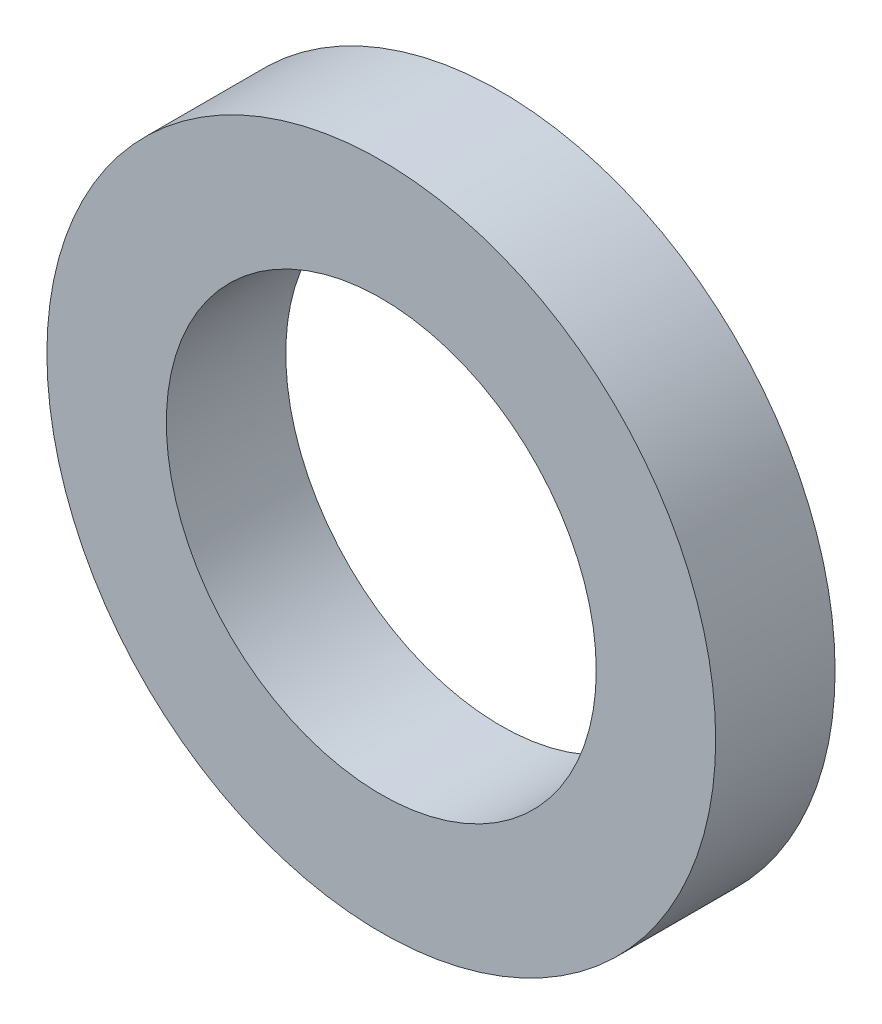
from build123d import *

# Parameters (mm, degrees)
SKETCH_1_R      = 140
SKETCH_1_R_2    = 90
EXTRUDE_1_DEPTH = 25


with BuildPart() as part:
    # 草图1 → 凸台-拉伸1 (new, symmetric)
    with BuildSketch(Plane.XY):
        Circle(SKETCH_1_R)
        Circle(SKETCH_1_R_2, mode=Mode.SUBTRACT)
    extrude(amount=EXTRUDE_1_DEPTH, both=True)


solid = part.part
